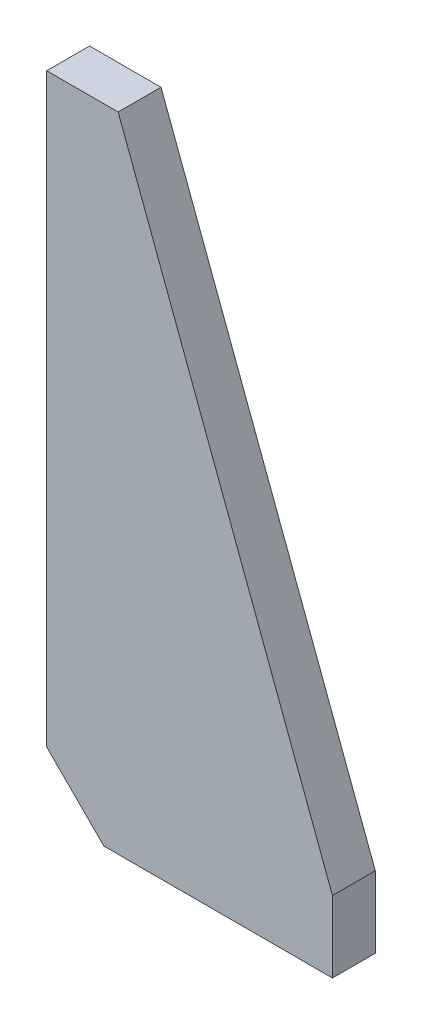
SolidWorks part; units mm, degrees
material "Q235B"
ref_plane "Front Plane" through (0, 0, 0) normal (0, 0, 1) x (1, 0, 0)
ref_plane "Top Plane" through (0, 0, 0) normal (0, 1, 0) x (1, 0, 0)
ref_plane "Right Plane" through (0, 0, 0) normal (1, 0, 0) x (0, 0, -1)
sketch "Sketch1" plane through (0, 0, 0) normal (0, 0, 1) x (1, 0, 0)
  line L0 (0, 90) -> (0, 0)
  line L1 (0, 0) -> (40, 0)
  line L2 (40, 0) -> (40, 10)
  line L3 (40, 10) -> (10, 90)
  line L4 (10, 90) -> (0, 90)
  dimension "D1" = 40
  dimension "D2" = 10
  dimension "D3" = 90
  dimension "D4" = 10
extrude "Boss-Extrude1" add sketch "Sketch1" along normal mid plane 6
chamfer "Chamfer1" distance 8 angle 45 1 edges at (0, 0, 0)
